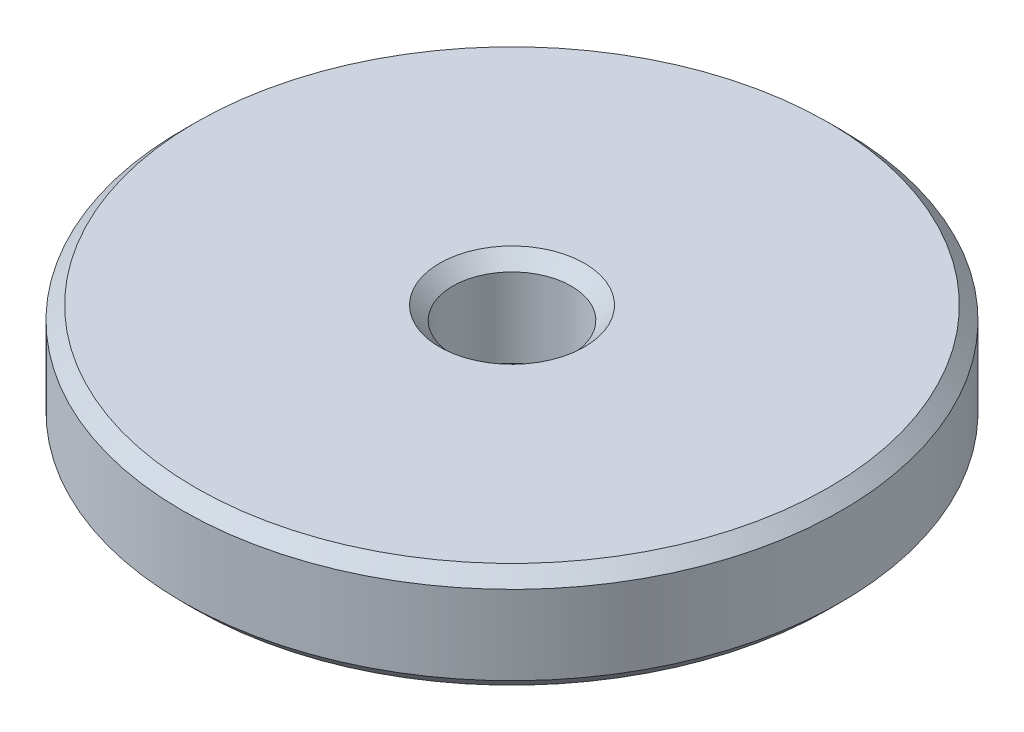
from build123d import *


with BuildPart() as part:
    # 草图1 → 旋转1 (revolve)
    with BuildSketch(Plane.XY, mode=Mode.PRIVATE) as revolve_1_sk:
        Polygon((24, 8), (5.5, 8), (4.5, 7), (4.5, 1), (5.5, 0), (24, 0), (25, 1), (25, 7), align=None)
    revolve(revolve_1_sk.sketch.rotate(Axis((0, 8, 0), (0, -1, 0)), 270), axis=Axis((0, 8, 0), (0, -1, 0)))


solid = part.part
